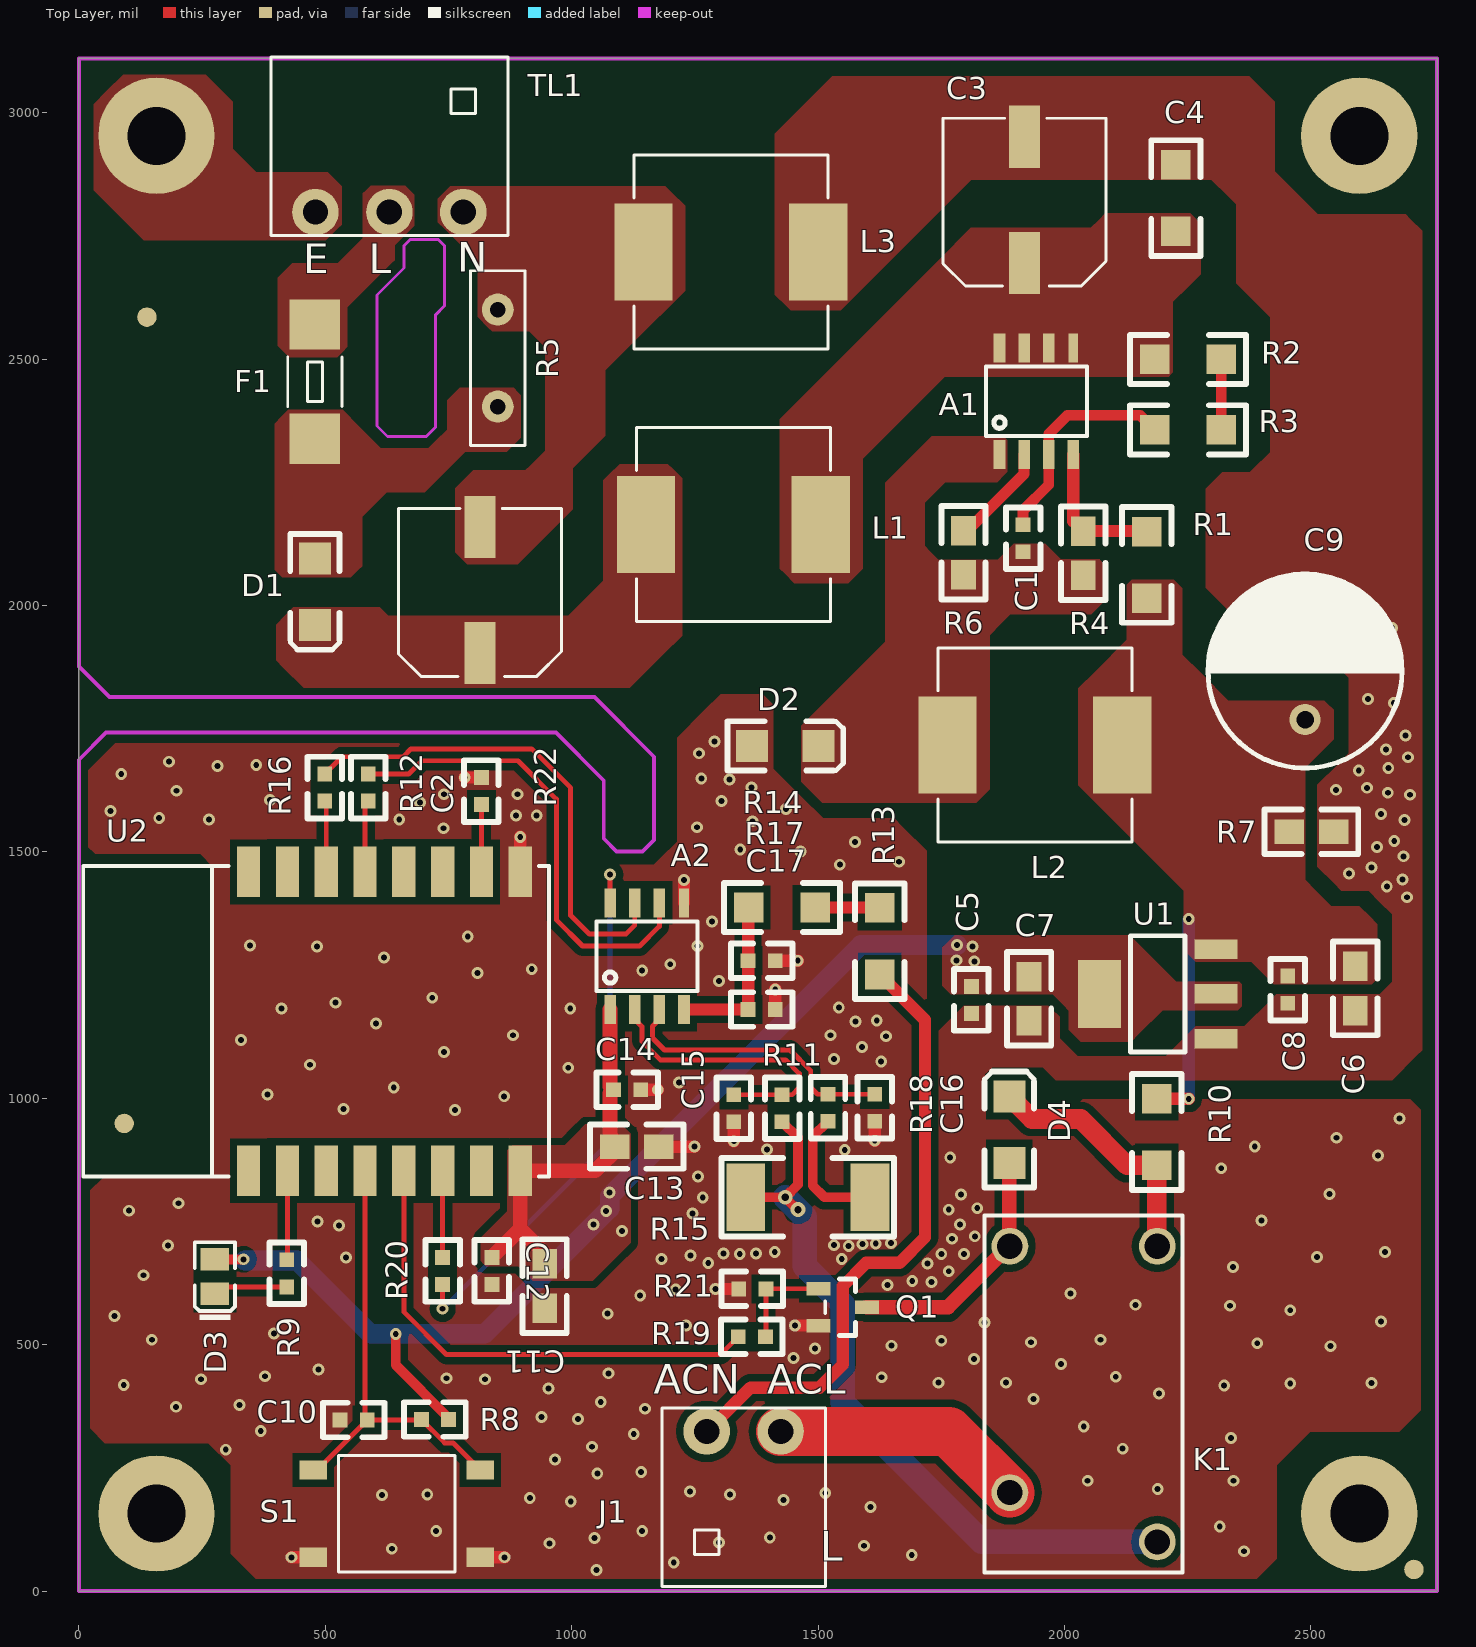
[diagram p0: Top Layer view]
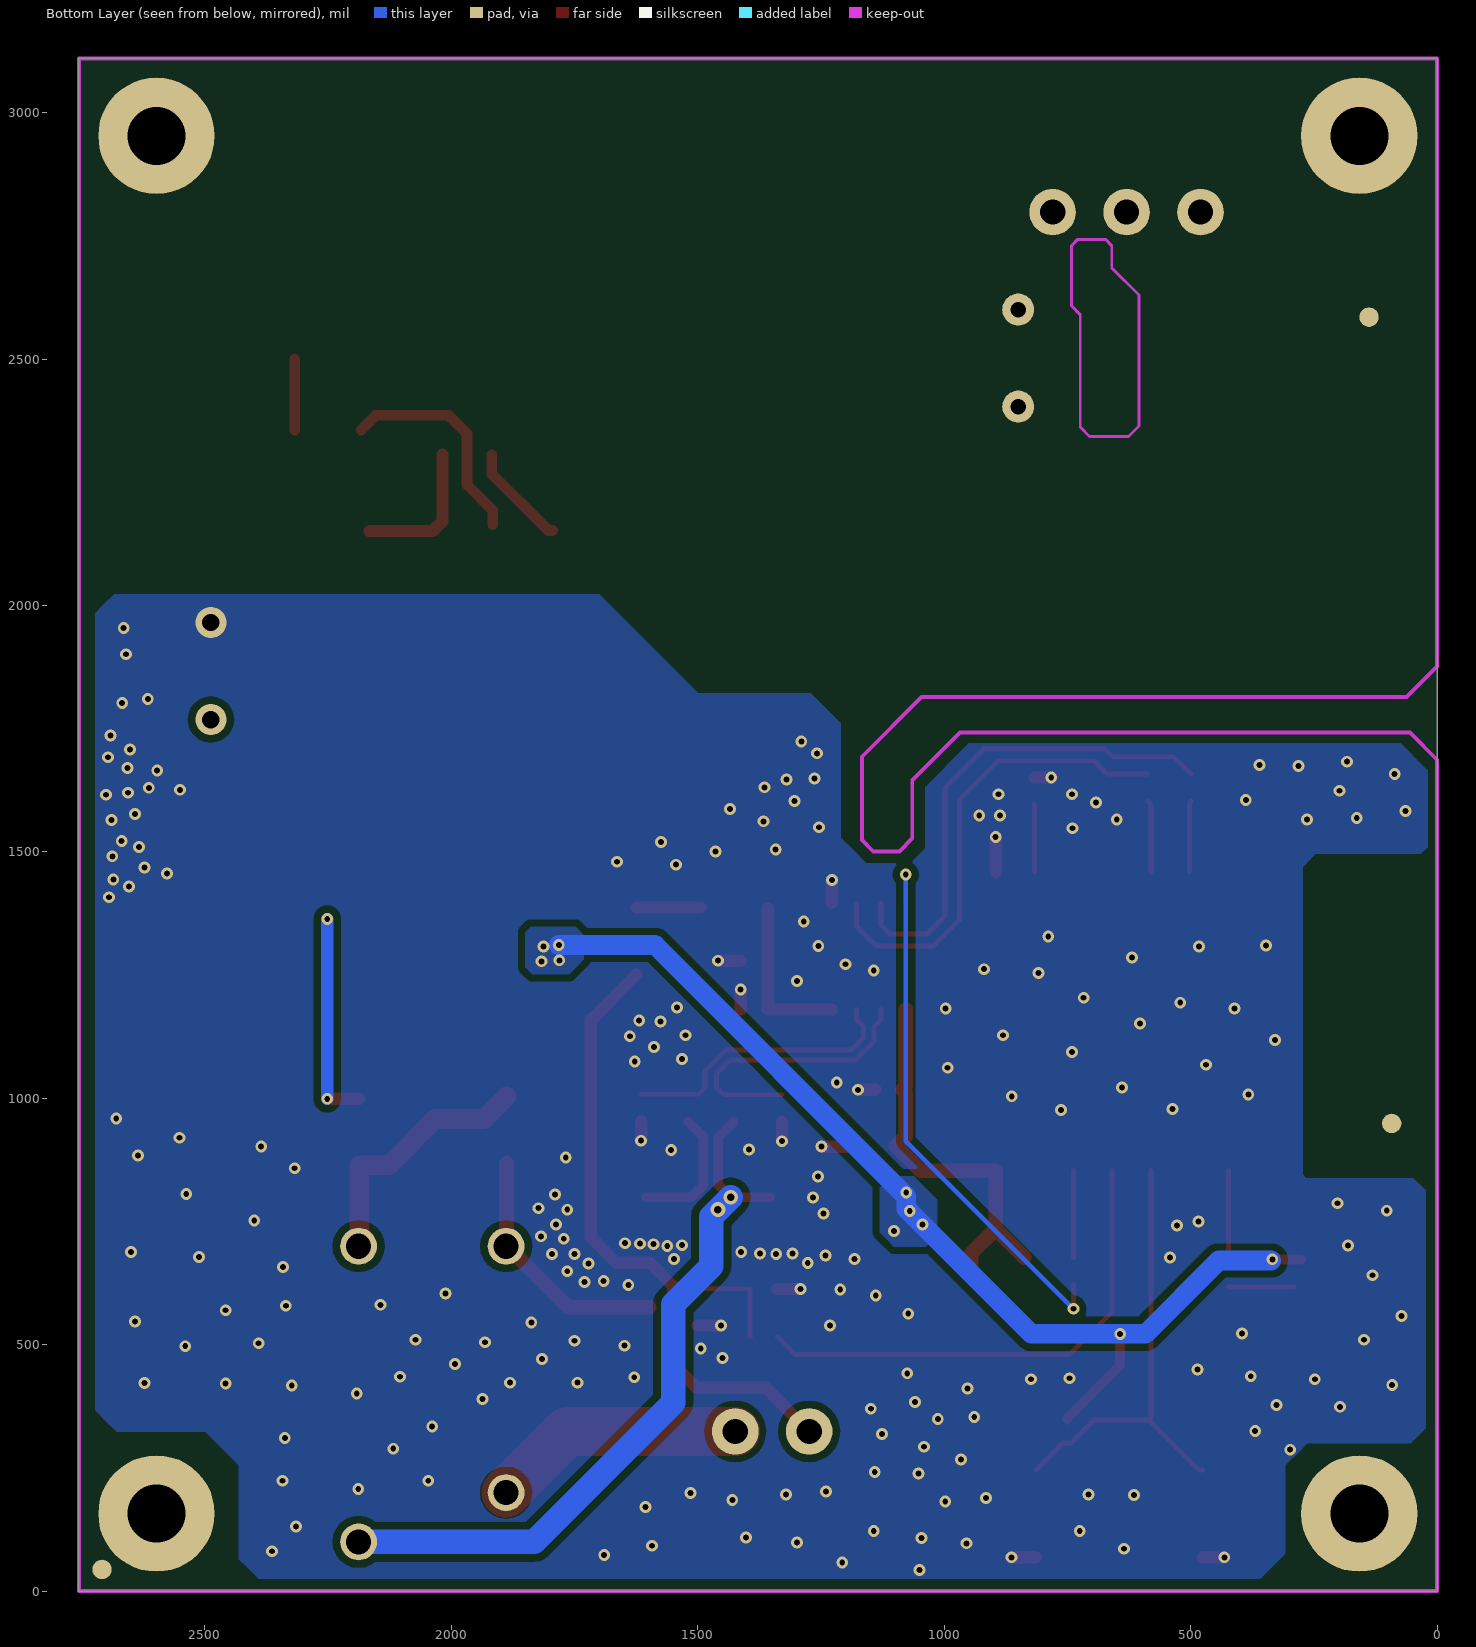
[diagram p1: Bottom Layer view, seen from below]
# Altium PCB MISC82282.PcbDoc
Units mil, origin at the board's own origin, x right, y up, seen from the top; angles counter-clockwise.
Board outline 2755.91 x 3110.24 mil, 2 copper layers (Top Layer, Bottom Layer); 56 components, 36 nets, 156 pads, 247 vias.

## Layer stack, top to bottom (the 12.6 mil dielectric is the usual default, probably not edited)
Top Layer: signal copper 1.4
Dielectric: dielectric 12.6, FR-4, Dk 4.8
Bottom Layer: signal copper 1.4

## Board outline
0,0 0,3110.24 2755.91,3110.24 2755.91,0

## Design rules (kind name [scope] priority, off if disabled: settings)
Clearance Clearance_1 [INPOLYGON] p1: gap=10
Clearance [All] p2: gap=10
DiffPairsRouting [All] p1: maxlimit=39.37 minlimit=6.06 mostfreqgap=10 maxuncoupledlength=500
HoleSize [All] p1: absolutevalues=TRUE maxlimit=500 minlimit=1 maxpercent=80.000 minpercent=20.000
HoleToHoleClearance [All] p1: gap=0 allowstackedmicrovias=TRUE
MinimumSolderMaskSliver [All] p1: minsoldermaskwidth=0
PlaneConnect [All] p1: planeconnectstyle=Relief reliefexpansion=20 reliefentries=4 reliefconductorwidth=19.68 reliefairgap=10
PolygonConnect PolygonConnect_1 [All vs ISVIA] p1: connectstyle=Direct reliefconductorwidth=10 reliefentries=4 polygonreliefangle="90 Angle"
PolygonConnect [All] p2: connectstyle=Direct reliefconductorwidth=20 reliefentries=4 polygonreliefangle="90 Angle"
RoutingVias [All] p1: holewidth=12 width=24 viastyle="Through Hole" minholewidth=12 minwidth=24 maxholewidth=12 maxwidth=24
SilkToSilkClearance [All] p1: silktosilkclearance=0
SilkscreenOverComponentPads SilkToSolderMaskClearance [IsPad] p1: minsilkscreentomaskgap=0
SolderMaskExpansion [All] p1: expansion=4
Width [All] p1: maxlimit=100 minlimit=10 preferedwidth=10 minimp=50.000000 maximp=50.000000 favimp=50.000000
21 further rules are at their usual default settings.

## Components (designator, comment, footprint, x,y, rotation, side; value= is the part's Value field where it differs from the comment)
A1 "SY50282" SO-8 1943,2414.23 r90 top
A2 "BL0937" SO-8 1153,1288.23 r90 top
C1 "2.2uF10% 50V" 0603 1916,2164 r270 top
C2 "3.3u/400V" SMD8x10.5 814,2031.23 r180 top
C3 "3.3u/400V" SMD8x10.5 1919,2823.23 r180 top
C4 "10nF10% 1kV" 1206 2226,2759 r90 top
C5 "100nF (104) 10% 50V" 0603 1811,1227 r270 top
C6 "10u/10V" 0805 2590,1268 r270 top
C7 "10u/10V" 0805 1928,1247 r270 top
C8 "100nF (104) 10% 50V" 0603 2453,1248 r270 top
C9 "680u/16V" 10X12.5 2488,1867 r270 top
C10 "100nF (104) 10% 50V" 0603 585,347.23 r180 top
C11 "10u/10V" 0805 945,664 r270 top
C12 "100nF (104) 10% 50V" 0603 838,677.23 r270 top
C13 "10u/10V" 0805 1087,902 r0 top
C14 "100nF (104) 10% 50V" 0603 1085,1017.23 r0 top
C15 "33nF 10% 50V" 0603 1329,1007.23 r270 top
C16 "33nF 10% 50V" 0603 1615,953.23 r90 top
C17 "33nF 10% 50V" 0603 1358,1180.23 r0 top
D1 "IN4007" SDIODE-2 479,1960.23 r90 top
D2 "SS34" SDIODE-2 1501,1715 r180 top
D3 "Green 0805" 0805_LED_S1 276,638.23 r90 top
D4 "IN4007" SDIODE-2 1888,1004 r270 top
F1 "MF2410F2.000TM" 2410 479,2454 r270 top
J1 "SIP2" DIP-2 1349,324 r0 top
K1 "HF32F-G/005-HS3" HF32F-G/005-HS3 2038.66,399.89 r270 top
L1 "VLP8040T-3R3N" IND10X10 1328,2164.23 r180 top
L2 "VLP8040T-3R3N" IND10X10 1940,1717 r180 top
L3 "VLP8040T-3R3N" IND10X10 1323,2717.23 r180 top
Q1 "S8050" SOT-23(SOT-23-3) 1550,576.23 r180 top
R1 "36K 1%" 1206 2167,2015 r90 top
R2 "1.5M 1%" 1206 2183,2499.23 r0 top
R3 "1.5M 1%" 1206 2318,2356.23 r180 top
R4 "10K 1%" 0805 2038,2151 r270 top
R5 "07d471K" 07d471K 850,2502 r270 top
R6 "0.9R 1%" 0805 1795,2152 r270 top
R7 "3.3K 1%" 0805 2456,1541 r0 top
R8 "10K" 0603 750,348.23 r180 top
R9 "2K" 0603 422,672.23 r270 top
R10 "330" 1206 2187,864 r90 top
R11 "1K 1%" 0603 1427,1007.23 r270 top
R12 "100R1%" 0603 587,1658 r270 top
R13 "1M1%" 1206 1625,1251.23 r90 top
R14 "1M1%" 1206 1494,1387.23 r180 top
R15 "1mR" 2512 1479,799.23 r90 top
R16 "100R1%" 0603 499,1658 r270 top
R17 "1K 1%" 0603 1358,1279.23 r0 top
R18 "1K 1%" 0603 1520,1008.23 r270 top
R19 "2K" 0603 1393,516.23 r180 top
R20 "100R1%" 0603 738,622.23 r90 top
R21 "10K" 0603 1394,613.23 r180 top
R22 "10K" 0603 816.85,1596 r90 top
S1 "SW-PB4P" smd6X6x4.5 645,157.23 r0 top
TL1 "SIP3" DIP-3 630,2798.23 r180 top
U1 "AMS1117-3.3" SOT-223 2189.12,1211.76 r90 top
U2 "WR3" WR3 620,1156.23 r90 top

## Footprints (in the part's own frame and the unit in brackets; to place one, negate y for a bottom-side part, rotate by r counter-clockwise, add the part's x,y. Pads: shape width x height; smd on the part's side, far side on the other; paste and mask are expansions set on the pad)
07d471K [mm]
  round 1.65 hole 0.8: 1(-2.5,0) 2(2.5,0)
  silkscreen extent -4.5,-1.4 4.5,1.4
10X12.5 [mm]
  round 1.6 hole 0.9: 1(2.5,0) 2(-2.5,0)
  silkscreen extent -5,-5 5,5, body extent -5,-4.99 5,4.99, height 14
0603 [mil]
  rect 30x30 smd: 1(0,0) 2(55,0)
  silkscreen extent -35,-35 90,35
0805 [mil]
  rect 60x50 smd: 1(0,0) 2(90,0)
  silkscreen extent -50,-45 140,45
0805_LED_S1 [mm]
  rect 1.16x1.47 smd: A(0.89,0) K(-0.89,0)
  silkscreen extent -2.24,-1.04 1.77,1.03, body extent -1.01,-0.63 1.01,0.62, height 1.1
1206 [mil]
  rect 60x60 smd: 1(0,0) 2(135,0)
  silkscreen extent -50,-50 185,50
2410 [mm]
  rect 2.6x2.6 smd: 1(-2.95,0) 2(2.95,0)
  silkscreen extent -1.27,-1.4 1.27,1.4
2512 [mm]
  rect 3.5x2 smd: 1(0,3.2) 2(0,-3.2)
  silkscreen extent -2.03,-4.44 2.03,4.45, body extent -1.6,-3.2 1.6,3.2, height 0.6
DIP-2 [mm]
  round 2.4 hole 1.3: 1(-1.905,0) 2(1.905,0)
  silkscreen extent -4.21,-8 4.21,1.2
DIP-3 [mm]
  round 2.4 hole 1.3: 1(-3.81,0) 2(0,0) 3(3.81,0)
  silkscreen extent -6.11,-8 6.11,1.2
HF32F-G/005-HS3 [mm]
  round 1.9 hole 1.3: 1(-7.62,3.8) 2(-7.62,-3.8) 3(7.62,3.8) 4(5.08,-3.8)
  silkscreen extent -9.2,-5.1 9.2,5.1
IND10X10 [mm]
  rect 3x5 smd: 1(-4.5,0) 2(4.5,0)
  silkscreen extent -5,-5 5,5
SDIODE-2 [mil]
  rect 65x65 smd: A(135,0) K(0,0)
  silkscreen extent -50,-50 185,50
smd6X6x4.5 [mm]
  rect 1.4x1 smd: 1(-4.3,2.25) 2(-4.3,-2.25) 3(4.3,-2.25) 4(4.3,2.25)
  silkscreen extent -3,-3 3,3
SMD8x10.5 [mm]
  rect 1.6x3.2 smd: 1(0,3.25) 2(0,-3.25)
  silkscreen extent -4.2,-4.2 4.2,4.45
SO-8 [mm]
  rect 1.5x0.6 smd: 1(-2.75,1.905) 2(-2.75,0.635) 3(-2.75,-0.635) 4(-2.75,-1.905) 6(2.75,-0.635) 7(2.75,0.635) 8(2.75,1.905)
  rect 1.5x0.5 smd: 5(2.75,-1.905)
  silkscreen extent -1.8,-2.6 1.8,2.6
SOT-23(SOT-23-3) [mm]
  rect 1.25x0.7 smd: 1(1.25,-0.95) 2(1.25,0.95) 3(-1.25,0)
  silkscreen extent -0.65,-1.46 0.9,1.46, body extent -1.5,-1.5 1.5,1.5, height 1.3
SOT-223 [mm]
  rect 1x2.2 smd: 1(-2.3,-3) 2(0,-3) 3(2.3,-3)
  rect 3.5x2.2 smd: 2(0,3)
  silkscreen extent -3,-1.4 3,1.4, body extent -3.24,-3.49 3.24,3.49, height 1.64
WR3 [mm]
  rect 2.6x1.2 smd: 1(-7.7,7) 2(-7.7,5) 3(-7.7,3) 4(-7.7,1) 5(-7.7,-1) 6(-7.7,-3) 7(-7.7,-5) 8(-7.7,-7) 9(7.7,-7) 10(7.7,-5) 11(7.7,-3) 12(7.7,-1) 13(7.7,1) 14(7.7,3) 15(7.7,5) 16(7.7,7)
  silkscreen extent -8,-8.48 8,15.52

## Part data
A1 A2: library part TPS54331DR
C1 C4 C10 C12 C14 C15 C16 C17: library part CAP, "Capacitor"
C2 C3 C6 C7 C9 C11 C13: library part ELECTRO1
C5 C8: library part "0603 100nF (104) 10% 50V", "SMD capacitor"
D1 D2 D4: library part DIODE, "Diode"
D3: library part "0805 翠绿", "LED"
F1: library part "Fuse Thermal", "Thermal Fuse"
K1: library part RELAY-SPST
L1 L2 L3: "Unknown"
Q1: library part NPN-1
R1 R2 R3 R4 R6 R7 R8 R10 R11 R12 R13 R14 R15 R16 R17 R18 R19 R20 R21 R22: library part RES2
R5: library part "Res Varistor", "Varistor (Voltage-Sensitive Resistor)"
R9: library part "0603 680Ω (6800) 1%", "SMD resistor"
S1: "6×6×5.0mm, black, SMD,,*"
U1: library part "SOT-223 AMS1117-3.3", "Low-dropout linear regulator (LDO)"
U2: library part SR_FRS_1WV

## Free pads (board coordinates)
  round 39.37 smd mask+39.37: 0(92,949) 0(138,2585) 0(2708.91,44)
  round 39.37 smd far side mask+39.37: 0(92,949) 0(138,2585) 0(2708.91,44)
  round 236.22 hole 118.11: 0(157.48,157.48) 0(157.48,2952.76) 0(2598.43,157.48) 0(2598.43,2952.76)

## Via types
v1: diameter 24, hole 12, Top Layer to Bottom Layer, 245 vias
v2: diameter 30, hole 15, Top Layer to Bottom Layer, 2 vias

## Nets (pads, with @x,y where several pads share a name; then routed paths per layer and width w, separated by ;. In a path a pad name is that pad's centre, name@x,y a point inside that pad or via, vN(x,y) a via of type N, cw(c..) or ccw(c..) an arc to the next point about the centre after c; other vN are vias at no path point)
+3.3V: A2.1 C5.1 C7.1 C11.1 C12.1 C13.1 C14.1 D3.A R8.1 U1.2 U2.8 | length 2929.5
  Top Layer w20: D3.A v1(334.27,673.27) ; v1(643,522) 643,458.51 750,351.51 R8.1
  Top Layer w30: C12.1 895.59,734.82 ; C11.1 945,685.41 895.59,734.82 ; A2.1 1078,1024.23 C14.1 1078,1010.23 1078,923.23 1098,903.23 1047.85,853.08 U2.8 895.59,734.82
  Bottom Layer w40: v1@337,671 443,671 592,522 823,522 1077,776 1077,801 1587,1311 v1(1782,1311)
  other v1: 1102,731 1044,744 1070,771 1077,809 1817,1278 1781,1280 1813,1308
+5V: C6.1 C8.1 C9.1 L2.1 R1.1 R7.1 R10.2 U1.3 | length 430
  Top Layer w25: R10.2 v1(2252,999)
  Bottom Layer w25: v1(2252,999) v1(2252,1364)
A5: R12.2 U2.13 | length 146.3
  Top Layer w10: U2.13 580.63,1596.63 R12.2
A12: R16.2 U2.14 | length 144.8
  Top Layer w10: R16.2 501.89,1600.11 U2.14
A14: R19.2 U2.5 | length 1016
  Top Layer w10: U2.5 659.37,566.63 746,480 1301.77,480 R19.2
A15: R20.2 U2.6 | length 175.7
  Top Layer w10: R20.2@738.11,677.34 U2.6
A19: C10.1 R8.2 S1.1 S1.4 U2.4 | length 929.7
  Top Layer w10: S1.1 483.58,245.81 C10.1 694,347.23 R8.2 742.23,301 759.1,301 S1.4 ; U2.4 580.63,351.6 C10.1@584,348.23
CF: A2.6 R12.1 | length 965.5
  Top Layer w10: R12.1 669,1658 696,1685 891,1685 969,1607 969,1362 1022,1309 1138,1309 1178,1349 A2.6
CF1: A2.7 R16.1 | length 1010.5
  Top Layer w10: R16.1 534,1693 658,1693 674,1709 919,1709 998,1630 998,1371 1036,1333 1110,1333 1128,1351 A2.7
CF1_S: A2.8 R20.1 | length 1128.6
  Top Layer w10: v1(738,573) R20.1 ; A2.8 v1(1078,1454)
  Bottom Layer w10: v1(738,573) 1078,913 v1(1078,1454)
EARTH: pad.0@157.48,2952.76 TL1.3
GND: A2.5 C3.2 C4.2 C5.2 C6.2 C7.2 C8.2 C9.2 C10.2 C11.2 C12.2 C13.2 C14.2 C15.2 C16.1 C17.2 D2.A L3.1 Q1.2 R7.2 R17.2 R21.2 R22.2 S1.2 S1.3 U1.1 U2.9 | length 611.6
  Top Layer w25: v1(431.65,68.65) S1.2 ; v1(782.85,1651) R22.2 ; S1.3 v1(863.65,68.65) ; U2.9 v1(895.59,1530.41) ; C14.2 v1(1174.77,1017.23) ; C13.2 v1(1249,902) ; A2.5 v1(1228,1443) ; v1(1291.77,613.23) R21.2 ; v1(1329,913) C15.2 ; C17.2 v1(1413,1221) ; R17.2 v1(1458.77,1279.23) ; v1(1453.17,538.83) Q1.2 ; v1(1615,914) C16.1
  other v1: 1050,43 1207,58 1690,73 2364,81 635,86 1593,92 955,97 1299,99 1046,108 1402,109 725,122 1143,122 2315,131 1606,171 998,182 1430,185 915,189 615,195 707,196 1321,196 1514.55,199 1240,202 2189,207 2047,224 2343,224 1052,239 1141,242 966,267 298,287 2118,289 1041,293 2338,311 1126,319 369,325 2039,334 1013,349 939,353 1149,370 197,374 326,378 1059,384 1937,390 2192,401 953,411 2324,417 91,418 2458,421 2623,422 1744,423 1881,423 248,430 824,430 746,432 1629,434 2104,435 378,436 1075,442 486,450 1993,461 1816,471 1450,473 1494,492 2540,497 1649,498 2391,503 1932,505 1750,508 148,510 2073,510 396,523 1232,539 1837.87,545 2642,547 72,558 1073,563 2458,570 2336,579 2144,581 1139,600 2012,604 1211,612 1641,621 1730,627 1691,629 131,641 1765,649 2342,658 1722,665 1277,666 1182,674 1548,674 542,677 2512,678 1241,681 1341,684 1750,684 1796,684 1308,685 1374,685 1412,688 2650,688 1562,700 181,701 1532,702 1590,704 1617,705 1648,706 1772,715 1818,720 528,742 1788,744 484,750 2400,752 1245,766 102,772 1765,774 1823,777 202,787 1266,799 1790,805 2538,806 1256,841 2318,858 1768,880 2636,884 1554,895 1396,896 2386,902 2552,920 2680,959 763,976 537,978 863,1004 383,1008 639,1022 1218,1032 993,1062 469,1068 1628,1075 1532,1080 741,1094 1589,1104 329,1118 1638,1126 881,1128 1525,1128 603,1152 1576,1156 1619,1158 411,1182 997,1182 1542,1184 521,1194 717,1204 1299,1238 809,1254 1143,1259 919,1262 1200,1272 619,1286 483,1308 1255.48,1309 347,1310 789,1328 1285,1359 2695,1408 2654,1430 2686,1444 2577,1456 2623,1468 1544,1474 1664,1480 2688,1491 1464,1501 1342,1505 2634,1510 1575,1520 2669,1522 740,1548 1254,1550 1367,1562 2690,1565 264,1566 650,1566 163,1569 887,1574 929,1574 2642,1577 64,1583 1435,1587 692,1600 1304,1603 388,1605 2701,1616 741,1617 890,1617 2656,1620 198,1624 2551,1626 2614,1630 1365,1631 1320,1647 1263,1649 86,1658 2597,1665 2657,1670 281,1674 360,1676 183,1683 2697,1692 1258,1700 2652,1708 1290,1724 2692,1736 2668,1802 2616,1810 2660,1901 2664.93,1954.25
GNDS: A1.1 C1.2 D2.K L2.2 R4.2 R6.2
L_OUT: J1.2 K1.4 | length 516.5
  Top Layer w100: J1.2 1764.94,324 K1.4
L_TO_R: K1.3 R11.2 R15.1 | length 1514.3
  Top Layer w20: R15.1 v2(1433.23,799.23) 1459,825 1459,920.23 R11.2 ; v2@1435,797 v2@1460.77,771.23
  Bottom Layer w50: v2(1433.23,799.23) 1473,759.46 1473,659 1550,582 1550,382 1832.11,99.89 K1.3
  other v2: 1459.23,774.23
N: J1.1 R13.1 | length 1270.5
  Top Layer w25: J1.1 1363,413 1503,413 1550,460 1550,618.71 1597.29,666 1665,666 1717,718 1717,1159.23 R13.1
NetA1_2: A1.2 R6.1 | length 209.6
  Top Layer w22: R6.1 1803,2152 1918,2267 A1.2
NetA1_3: A1.3 C1.1 R3.2 | length 448.6
  Top Layer w22: C1.1 1916,2193 1968,2245 A1.3 1968,2348 2006,2386 2153.23,2386 R3.2
NetA1_4: A1.4 R1.2 R4.1 | length 292.7
  Top Layer w22: R1.2@2166,2151 R1.2
  Top Layer w25: A1.4 2018,2171 R4.1 R1.2@2166,2151
NetA1_5: A1.5 A1.6 A1.7 A1.8 C3.1 C4.1 L1.1 R2.1
NetC2_1: C2.1 D1.K L1.2
NetC2_2: C2.2 L3.2 R5.1 TL1.1
NetD1_A: D1.A F1.2 R5.2
NetD3_K: D3.K R9.2 | length 132
  Top Layer w10: D3.K@290.04,617.23 R9.2
NetD4_A: D4.A K1.2 Q1.3 | length 508.5
  Top Layer w30: Q1.3 1763.28,576.23 1888,700.94 D4.A
NetD4_K: D4.K K1.1 R10.1 | length 519.8
  Top Layer w40: D4.K 1934,958 2033,958 2127,864 R10.1 K1.1@2187,701.16
NetF1_1: F1.1 TL1.2
NetQ1_1: Q1.1 R19.1 R21.1 | length 204.4
  Top Layer w10: R19.1 1394,517.23 R21.1 1394.4,613.63 Q1.1
NetR2_2: R2.2 R3.1 | length 143
  Top Layer w22: R3.1 R2.2
NetR13_2: R13.2 R14.1 | length 131.4
  Top Layer w20: R13.2@1624,1387.23 R13.2
  Top Layer w25: R14.1 R13.2@1624,1387.23
NetR15_2: R15.2 R18.2 | length 268.9
  Top Layer w20: R18.2 1489,922.23 1489,823 1512.77,799.23 R15.2
NetR22_1: R22.1 U2.10 | length 136.6
  Top Layer w10: U2.10 R22.1
V1N: A2.3 C16.2 R18.1 | length 581.6
  Top Layer w10: A2.3 1178,1160 1164,1146 1164,1122.28 1188.28,1098 1443,1098 1485,1056 1485,1022 1498.77,1008.23 R18.1 C16.2
V1P: A2.2 C15.1 R11.1 | length 584.2
  Top Layer w10: A2.2 1128,1160 1142.36,1145.64 1142.36,1115.64 1180,1078 1434,1078 1462,1050 1462,1022 1447.23,1007.23 R11.1 C15.1
V2P: A2.4 C17.1 R14.2 R17.1 | length 437.3
  Top Layer w10: C17.1@1357.73,1179.96 C17.1 R17.1 ; R14.2@1358,1386.23 R14.2
  Top Layer w20: R14.2@1357.73,1385.96 R14.2@1358,1386.23
  Top Layer w25: A2.4 1228.27,1180.23 C17.1 R17.1 R14.2@1358,1386.23
WIFI_LED1: R9.1 U2.2 | length 181.3
  Top Layer w10: R9.1 423.15,673.38 U2.2
pads on no net: U2.1 U2.3 U2.7 U2.11 U2.12 U2.15 U2.16

## Polygon pours and split planes (outlines as drawn)
+3.3V on Top Layer "Top Layer-No Net" (solid, remove dead copper, pour order 1000): 1752,1294 1752,1246 1752,1228 1761,1219 1769,1211 1817,1211 1976,1211 1997,1190 2009,1178 2009,1158 2009,1139 2023,1125 2033,1115 2052,1115 2135,1115 2151,1131 2199,1179 2299,1179 2352,1179 2357,1184 2360,1187 2360,1198 2360,1231 2357,1234 2355,1236 2347,1236 2227,1236 2196,1267 2132,1331 2014,1331 1777,1331 1761,1315 1752,1306 1752,1294
+3.3V on Top Layer "Top Layer-No Net" (solid, remove dead copper, pour order 1001): 869,877 869,771 853,755 815,717 815,684 815,670 822,663 826,659 853,659 892,659 921,630 999,630 1043,630 1084,671 1120,707 1120,862 1120,928 1113,935 1101,947 1080,947 1028,947 1009,928 986,905 923,905 879,905 872,898 869,895 869,877
+5V on Top Layer "Top Layer-No Net" (solid, remove dead copper, pour order 1002): 2126,2029 2126,1930 2062,1866 2028,1832 2028,1753 2028,1635 2088,1575 2242,1421 2242,1364 2242,1301 2263,1280 2266,1277 2302,1277 2379,1277 2405,1251 2425,1231 2466,1231 2623,1231 2635,1243 2635,1280 2635,1353 2619,1369 2598,1390 2571,1390 2541,1390 2510,1421 2488,1443 2488,1538 2488,1670 2488,1671 2545,1728 2546,1729 2546,1763 2546,1788 2531,1803 2527,1807 2496,1807 2332,1807 2277,1862 2239,1900 2239,1997 2239,2035 2228,2046 2222,2052 2194,2052 2136,2052 2129,2045 2126,2042 2126,2029
GNDS on Top Layer "Top Layer-No Net" (solid, remove dead copper, pour order 1003): 1466,1756 1466,1642 1487,1621 1508,1600 1667,1600 1821,1600 1833,1612 1848,1627 1848,1913.85 1848,1940 1872,1964 1890,1982 1969,1982 2054,1982 2069,1997 2083,2011 2083,2038 2083,2082 2073,2092 2071,2094 1992,2094 1970,2116 1961,2125 1937,2125 1897,2125 1881,2109 1865,2093 1823,2093 1744,2093 1728,2109 1716,2121 1716,2151 1716,2208 1736,2228 1758,2250 1852,2250 1863,2250 1879,2266 1884,2271 1884,2291 1884,2335.46 1876,2343.46 1840.5,2343.46 1730.46,2343.46 1684,2297 1636,2249 1636,2143 1636,1926 1466,1756
NetA1_5 on Top Layer "Top Layer-No Net" (solid, remove dead copper, pour order 1004): 1422,2243 1422,2075 1433,2064 1452,2045 1489,2045 1561,2045 1576,2060 1591,2075 1591,2099 1591,2298 1672,2379 1757,2464 2169,2464 2211,2464 2216,2469 2220,2473 2220,2493 2220,2616 2251,2647 2276,2672 2276,2723 2276,2775 2255,2796 2212,2796 2083,2796 2069,2782 2053,2766 1949,2766 1810,2766 1745,2701 1422,2378 1422,2243
NetC2_2 on Top Layer "Top Layer-No Net" (solid, remove dead copper, pour order 1005): 728,2816 728,2778 743,2763 806,2700 809,2697 809,2591 809,2586 832,2563 839,2556 872,2556 914,2556 932,2538 946,2524 946,2354 946,2314 916,2284 906,2274 857,2274 800,2274 786,2260 764,2238 764,2196.58 764,2108 779,2093 788,2084 831,2084 891,2084 933,2126 1002,2195 1002,2251 1002,2278 1034,2310 1068,2344 1068,2438 1068,2476.85 1126.15,2535 1230,2638.85 1230,2802 1230,2811 1201,2840 1190,2851 1147,2851 754,2851 740,2837 728,2825 728,2816
NetF1_1 on Top Layer "Top Layer-No Net" (solid, remove dead copper, pour order 1006): 576,2827 576,2768 576,2745 559,2728 525,2694 478,2694 433,2694 415,2676 404,2665 404,2617 404,2527 414,2517 427,2504 457,2504 524,2504 535,2515 545,2525 545,2547 545,2605 635,2695 641,2701 641,2727 641,2730.98 661,2750.98 681,2770.98 681,2805 681,2833 668,2846 662,2852 635,2852 592,2852 582,2842 576,2836 576,2827
NetD1_A on Top Layer "Top Layer-No Net" (solid, remove dead copper, pour order 1007): 397,2328 397,2073 413,2057 508,2057 552,2057 567,2072 575,2080 575,2113 575,2180 596,2201 625,2230 683,2230 702,2230 730,2258 784,2312 829,2312 868.17,2312 881,2324.83 897,2340.83 897,2372 897,2427 891,2433 882,2442 870,2442 773,2442 763,2432 747,2416 747,2399 747,2357 723,2333 709,2319 670,2319 613,2319 568,2364 535,2397 500,2397 425,2397 411,2383 397,2369 397,2328
EARTH on Top Layer "Top Layer-No Net" (solid, remove dead copper, pour order 1008): 30,2990 30,2843 80,2793 132,2741 478,2741 501,2741 524,2764 533,2773 533,2802 533,2851 515,2869 505,2879 445,2879 360,2879 338,2901 312,2927 312,2963 312,3022 295,3039 257,3077 187,3077 90,3077 57,3044 30,3017 30,2990
NetC2_1 on Top Layer "Top Layer-No Net" (solid, remove dead copper, pour order 1009): 400,1952 400,1889 414,1875 456,1833 828,1833 1118,1833 1185,1900 1224,1939 1224,2084 1224,2258 1205,2277 1195,2287 1118,2287 1097,2287 1075,2265 1064,2254 1064,2218 1064,2050 1036,2022 993,1979 837,1979 628,1979 620,1987 611,1996 579,1996 435,1996 419,1980 400,1961 400,1952
GND on Top Layer "Top Layer-No Net" (solid, remove dead copper, pour order 1010): 1412,2841 1412,2631 1436,2607 1444,2599 1484,2599 1546,2599 1573,2626 1811,2864 2216,2864 2298,2864 2333,2829 2348,2814 2348,2770 2348,2654 2406,2596 2417,2585 2417,2516 2417,2311 2382,2276 2376,2270 2337,2270 2320,2270 2299,2249 2287,2237 2287,2163 2287,2036 2374,1949 2413,1910 2487,1910 2520,1910 2551,1879 2577,1853 2577,1804 2577,1700 2556,1679 2513,1636 2513,1560 2513,1470 2547,1436 2562,1421 2584,1421 2617,1421 2640,1398 2665,1373 2665,1259 2665,1236 2648,1219 2640,1211 2608,1211 2430,1211 2418,1199 2365,1146 2337,1146 2266.24,1146 2205.24,1085 2098,1085 2027,1085 1998,1114 1990,1122 1990,1143 1990,1165 1973,1182 1967,1188 1949,1188 1796,1188 1761,1153 1723,1115 1723,1012 1723,725 1684,686 1651,653 1651,637 1651,625 1659,617 1663,613 1694,613 1735,613 1767,645 1818,696 1818,736 1818,1028 1842,1052 1853,1063 1919,1063 1956,1063 1968,1051 1982,1037 2181,1037 2665,1037 2714,1086 2726,1098 2726,1183 2726,2760 2701,2785 2692,2794 2649,2794 2514,2794 2458,2850 2427,2881 2427,2955 2427,3022 2391,3058 2375,3074 2269,3074 1529,3074 1473,3018 1412,2957 1412,2841
GND on Top Layer "Top Layer-No Net" (solid, remove dead copper, pour order 1011): 15,1661 15,1514 32,1497 33,1496 246,1496 272.14,1469.86 273,1469 273,1445.42 273,846 265,838 48,838 23,813 23,790 23,330 53,300 99,300 263,300 308,255 308,247.7 308,76 359,25 368,25 2389.92,25 2431,66.08 2431,246.07 2431,255 2499,323 2679,323 2720.83,364.83 2723,367 2723,374 2723,977 2712,988 2702,998 2608,998 1888,998 1792,1094 1720,1166 1720,1410 1720,1502 1672,1550 1654,1568 1580,1568 1510,1568 1465,1613 1409,1669 1409,1743 1409,1799 1396,1812 1388,1820 1366,1820 1302,1820 1269,1787 1214,1732 1214,1670 1214,1521 1181,1488 1167,1474 1120,1474 1072,1474 1039,1507 1039,1535 1039,1635 977,1697 954,1720 74,1720 15,1661
+3.3V on Bottom Layer "Top Layer-No Net" (solid, remove dead copper, pour order 1012): 1731,1311 1731,1282 1741,1272 1761,1252 1790,1252 1836,1252 1846,1262 1850,1266 1850,1298 1850,1337 1842,1345 1839,1348 1815,1348 1748,1348 1739,1339 1731,1331 1731,1311
+3.3V on Bottom Layer "Top Layer-No Net" (solid, remove dead copper, pour order 1013): 1014,755 1014,722 1027,709 1037,699 1073,699 1102,699 1120,717 1131,728 1131,777 1131,818 1117,832 1107,842 1086,842 1062,842 1048,828 1014,794 1014,755
GND on Bottom Layer "Top Layer-No Net" (solid, remove dead copper, pour order 1014): 15,1645 15,1514 32,1497 33,1496 112,1496 246,1496 255,1487 273,1469 273,1443 273,846 267,840 265,838 239,838 48,838 27,817 23,813 23,777 23,330 46,307 53,300 99,300 263,300 279,284 308,255 308,164 308,76 327,57 359,25 487,25 2391,25 2413,47 2431,65 2431,170 2431,255 2468,292 2499,323 2589,323 2679,323 2698,342 2723,367 2723,419 2723,1618 2723,1984 2706,2001 2684,2023 2505,2023 1709,2023 1700,2023 1558,1881 1499,1822 1385,1822 1271,1822 1248,1799 1210,1761 1210,1690 1210,1529 1184,1503 1158,1477 1146,1477 1069,1477 1062,1484 1039,1507 1039,1525 1039,1625 1039,1631 958,1712 950,1720 927,1720 74,1720 26,1672 15,1661 15,1645

## Keep-outs
Keep-Out Layer:
  lines w5.91: 0,1876 0,1887 ; 605,2364 605,2630 660,2685 660,2730 673,2743 729,2743 742,2730 742,2608 724,2590 724,2362 705,2343 626,2343 605,2364
  lines w7.87: 0,0 2755.91,0 2755.91,3110.24 0,3110.24 0,1876 62,1814 1046,1814 1167,1693 1167,1524 1144,1501 1091,1501 1065,1527 1065,1645 968,1742 55,1742 0,1687 0,0

## Silkscreen, mask and mechanical layers (free items; w line width, h text height)
Top Overlay:
  text "N" at 768,2677 h60
  text "E" at 455,2674 h60
  text "L" at 588,2674 h60
  text "ACN" at 1166,401 h60
  text "ACL" at 1397,400 h60
  text "L" at 1504,62 h60